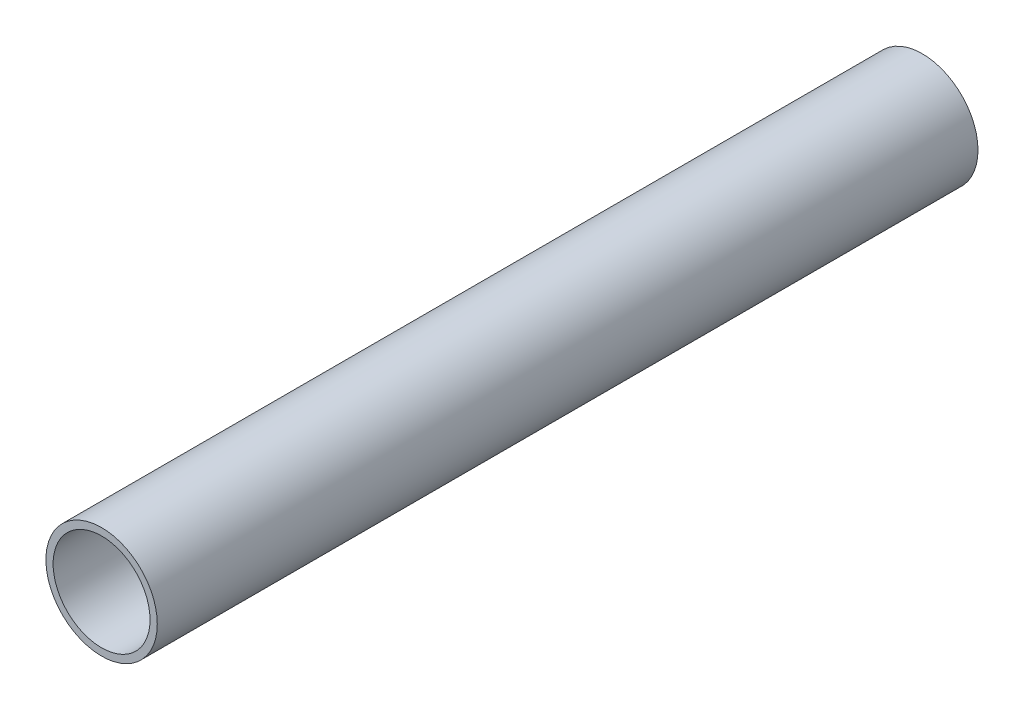
SolidWorks part; units mm, degrees
ref_plane "Front Plane" through (0, 0, 0) normal (0, 0, 1) x (1, 0, 0)
ref_plane "Top Plane" through (0, 0, 0) normal (0, 1, 0) x (1, 0, 0)
ref_plane "Right Plane" through (0, 0, 0) normal (1, 0, 0) x (0, 0, -1)
sketch "Sketch1" plane through (0, 0, 0) normal (0, 0, 1) x (1, 0, 0)
  circle A0 centre (0, 0) radius 30.1625
  circle A1 centre (0, 0) radius 26.2509
extrude "Boss-Extrude1" add sketch "Sketch1" along normal up to vertex (222.25 mm away) and the other way up to vertex (222.25 mm away)
